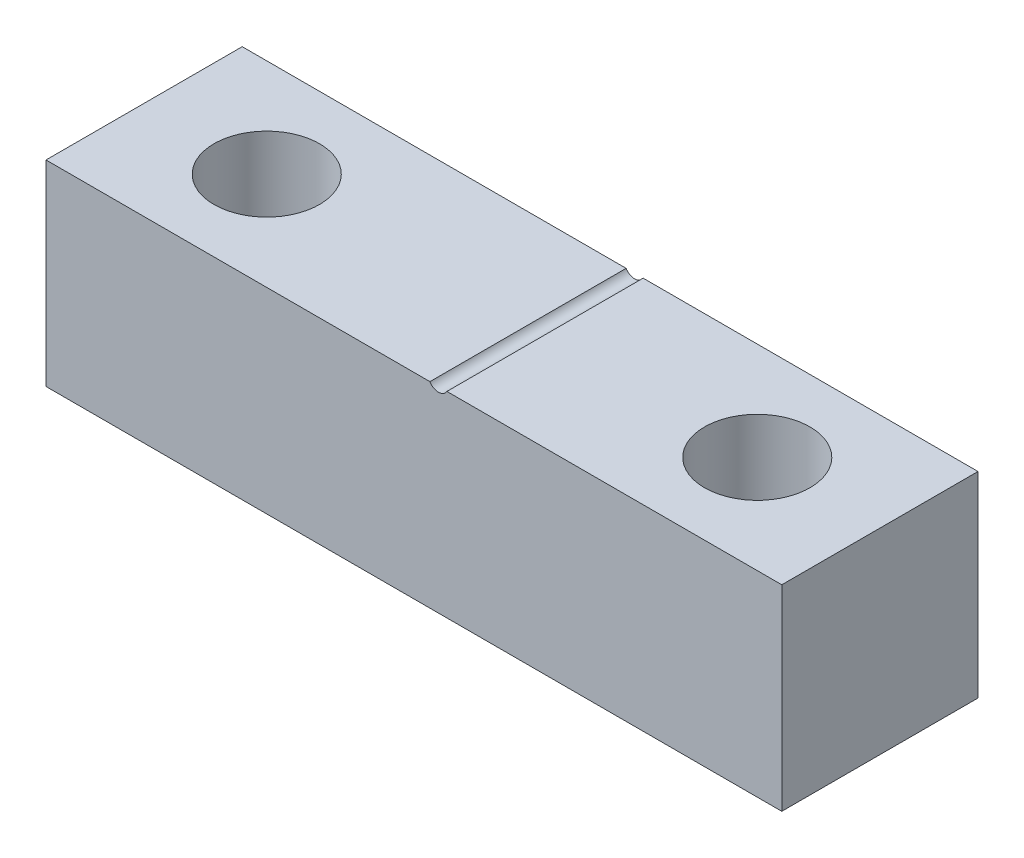
from build123d import *

# Parameters (mm, degrees)
SKETCH_1_W          = 30
SKETCH_1_H          = 8
EXTRUDE_1_DEPTH     = 8
SKETCH_2_R          = 2.15
CUT_EXTRUDE_1_DEPTH = 21.498011819
CUT_EXTRUDE_2_DEPTH = 20.588803717


with BuildPart() as part:
    # 草图1 → 凸台-拉伸1 (new body)
    with BuildSketch(Plane.XY):
        with Locations((2.092936803, -1.249070632)):
            Rectangle(SKETCH_1_W, SKETCH_1_H)
    extrude(amount=EXTRUDE_1_DEPTH)

    # 草图2 → 切除-拉伸1 (cut, through all)
    with BuildSketch(Plane(origin=(0, 2.750929368, 0), x_dir=(1, 0, 0), z_dir=(0, 1, 0))):
        with Locations(Location((-7.907063197, -4, 0), (0, 0, 270))):
            Circle(SKETCH_2_R)
        with Locations(Location((12.092936803, -4, 0), (0, 0, 270))):
            Circle(SKETCH_2_R)
    extrude(amount=-CUT_EXTRUDE_1_DEPTH, mode=Mode.SUBTRACT)

    # 草图3 → 切除-拉伸2 (cut, through all)
    with BuildSketch(Plane.XY.offset(8)):
        with BuildLine():
            Line((2.746526641, 2.750929368), (3.439346964, 2.750929368))
            ThreePointArc((3.439346964, 2.750929368), (3.092936803, 2.550929368), (2.746526641, 2.750929368))
        make_face()
    extrude(amount=-CUT_EXTRUDE_2_DEPTH, mode=Mode.SUBTRACT)


solid = part.part
